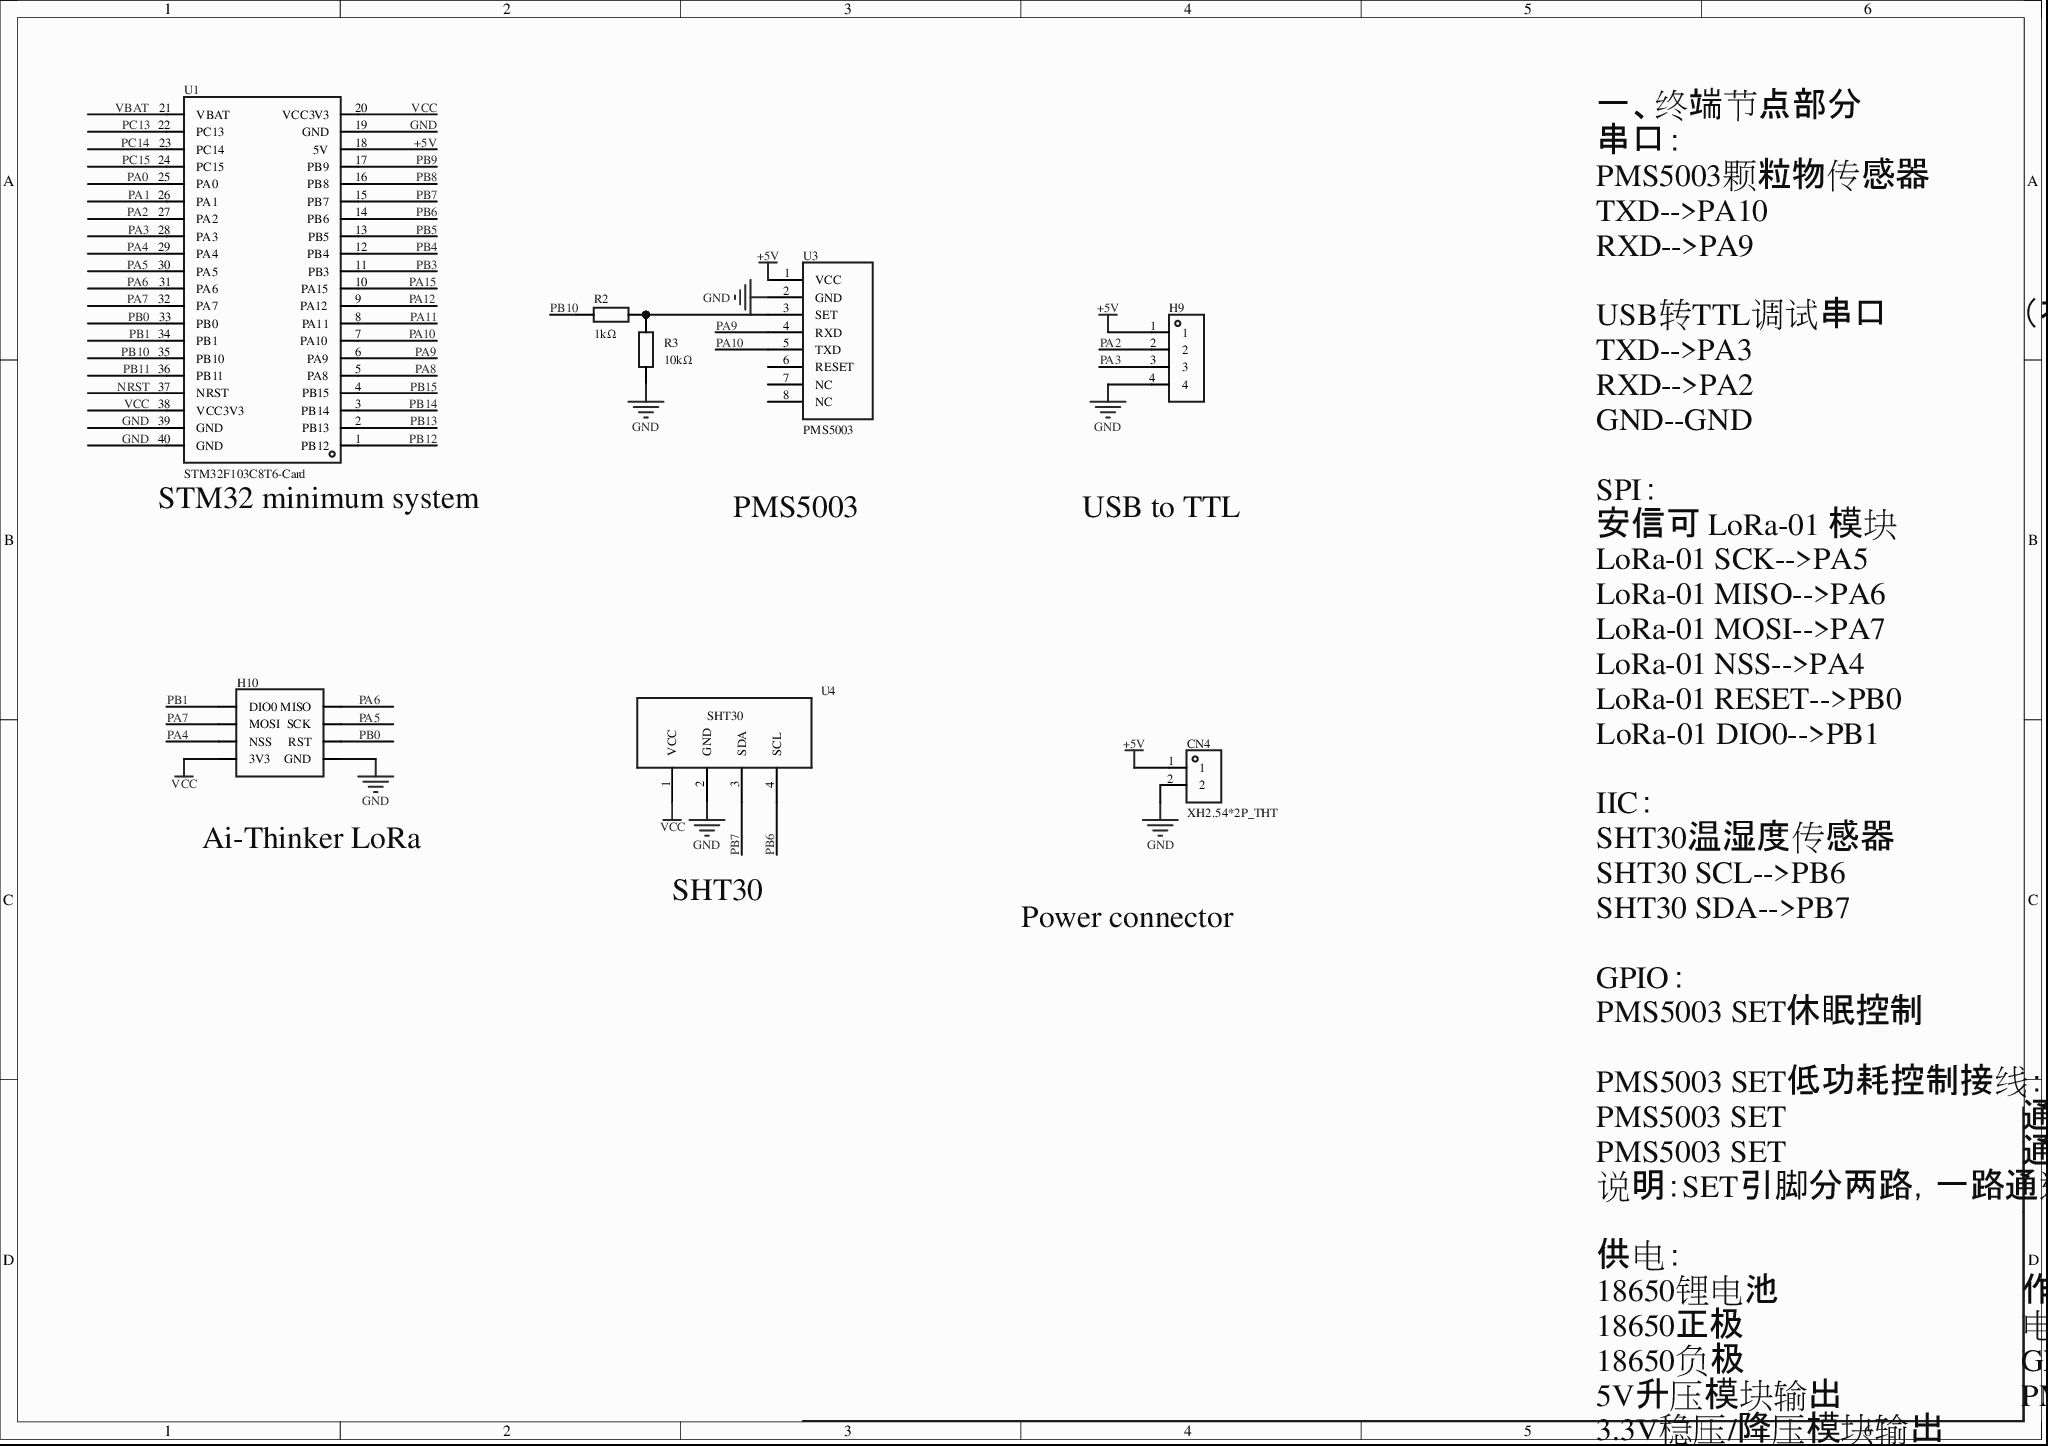
[diagram p0: MISC88998-3.schdoc]
# Altium project MISC88998-2.PrjPcb
1 sheet, 8 parts. Net scope: global (net labels, ports and power ports of the same name join across sheets).
Board file: MISC88998.pcbdoc

## Sheet MISC88998-3.schdoc
size 297 x 209 mm; Version: V1.0; @Project Name: MISC88998; @Page Count: 1; @Update Date: 2026-05-13; @Create Date: 2026-05-13; @Schematic Name: MISC88998; @Page No: 1; @Create Time: 23:22:16; @Update Time: 17:32:40; @Board Name: MISC88998

### Parts
CN4  XH2.54*2P_THT  [CONN-TH_2P-P2.50-XH2.54-2P]
H9  (no value)  [HDR-TH_4P-P2.54-V-M]
H10  (no value)  [HDR-TH_8P-P2.54-V-F-R2-C4-S2.54-1]
R2  1kΩ  [Res_1/8W]
R3  10kΩ  [Res_1/8W]
U1  STM32F103C8T6-Card  [CONN-TH_L53.3-W22.9_STM32F103C8T6-CARD]
U3  PMS5003  [1.25-LI-8P]
U4  (no value)  [SHT30模块]

### Nets
+5V: CN4.1 H9.1 U1.18(5V) U3.1(VCC)
GND: CN4.2 H9.4 H10.8(GND) R3.1 U1.19(GND) U1.39(GND) U1.40(GND) U3.2(GND) U4.2(GND)
VCC: H10.7(3V3) U1.20(VCC3V3) U1.38(VCC3V3) U4.1(VCC)
NRST: U1.37(NRST)
PA0: U1.25(PA0)
PA1: U1.26(PA1)
PA2: H9.2 U1.27(PA2)
PA3: H9.3 U1.28(PA3)
PA4: H10.5(NSS) U1.29(PA4)
PA5: H10.4(SCK) U1.30(PA5)
PA6: H10.2(MISO) U1.31(PA6)
PA7: H10.3(MOSI) U1.32(PA7)
PA8: U1.5(PA8)
PA9: U1.6(PA9) U3.4(RXD)
PA10: U1.7(PA10) U3.5(TXD)
PA11: U1.8(PA11)
PA12: U1.9(PA12)
PA15: U1.10(PA15)
PB0: H10.6(RST) U1.33(PB0)
PB1: H10.1(DIO0) U1.34(PB1)
PB3: U1.11(PB3)
PB4: U1.12(PB4)
PB5: U1.13(PB5)
PB6: U1.14(PB6) U4.4(SCL)
PB7: U1.15(PB7) U4.3(SDA)
PB8: U1.16(PB8)
PB9: U1.17(PB9)
PB10: R2.1 U1.35(PB10)
PB11: U1.36(PB11)
PB12: U1.1(PB12)
PB13: U1.2(PB13)
PB14: U1.3(PB14)
PB15: U1.4(PB15)
PC13: U1.22(PC13)
PC14: U1.23(PC14)
PC15: U1.24(PC15)
VBAT: U1.21(VBAT)
NetR2_2: R2.2 R3.2 U3.3(SET)

Not connected (* = marked no-connect by the designer): U3 6(RESET) 7(NC) 8(NC)

### Notes on the sheet
- 一、终端节点部分
  串口：
  PMS5003颗粒物传感器
  TXD-->PA10
  RXD-->PA9
  USB转TTL调试串口	（有单独模块不用画进PCB，给我留个接口即插即用）
  TXD-->PA3
  RXD-->PA2
  GND--GND
  SPI：
  安信可 LoRa-01 模块
  LoRa-01 SCK-->PA5
  LoRa-01 MISO-->PA6
  LoRa-01 MOSI-->PA7
  LoRa-01 NSS-->PA4
  LoRa-01 RESET-->PB0
  LoRa-01 DIO0-->PB1
  IIC：
  SHT30温湿度传感器
  SHT30 SCL-->PB6
  SHT30 SDA-->PB7
  GPIO：
  PMS5003 SET休眠控制		PB10
  PMS5003 SET低功耗控制接线：
  PMS5003 SET		通过1kΩ电阻接 STM32 PB10
  PMS5003 SET		通过10kΩ电阻接 GND
  说明：SET引脚分两路，一路通过1kΩ接PB10，另一路通过10kΩ接GND。PB10输出高电平时PMS5003工作，PB10输出低电平时PMS5003休眠；10kΩ下拉用于保证上电默认休眠。
  供电：
  18650锂电池		作为终端节点主电源
  18650正极		电源开关		系统电源输入
  18650负极		GND
  5V升压模块输出		PMS5003 VCC
  3.3V稳压/降压模块输出		STM32、SHT30、LoRa-01
  所有模块GND		公共GND
  说明：PMS5003由升压后的5V供电；STM32、SHT30和LoRa-01由稳定3.3V供电，LoRa-01不能接5V。
  电源滤波：
  LoRa-01 VCC 与 GND之间		并联10μF和0.1μF电容
  PMS5003 VCC 与 GND之间		并联100μF和0.1μF电容
  SWD下载接口：
  我的最小开发板上有，应该可以不用多做
- (near U1) STM32 minimum system
- PMS5003
- USB to TTL
- (near H10) Ai-Thinker LoRa
- SHT30
- Power connector

### Library data of the parts
CN4 = XH2.54*2P_直插: AddInBom: yes; ModelId: 325c595e30db4df8abe76612dd40b0fa0819f05c4eef4c71ace90d822a990e87; ModelTransform: 295.275,228.346,0,180,0,0,-0.002,-20.079,-137.795; Device: XH2.54*2P_THT; Symbol: XH2.54*2P_THT; FootprintName: CONN-TH_2P-P2.50-XH2.54-2P; LCSC Part Name: XH2.54*2P_直插; SupplierPart: C9900008615; ManufacturerPart: XH2.54*2P_直插; Supplier Footprint: XH2.54_2P; JLCPCB Part Class: Extended Part; Supplier: LCSC; ConvertToPcb: yes; ModelName: CONN-TH_2P-P2.50-XH2.54-2P
H9 = HDR-M_2.54_1x4P: Symbol: PZ254V-11-04P; ConvertToPcb: yes; ModelId: 112f4d05e8d64e99ab9a333894bea4f90819f05c4eef4c71ace90d822a990e87; ModelName: HDR-TH_4P-P2.54-M-LI-1X4P; ModelTransform: 399.999,104.7242,0,0,0,0,0,0,-118.11; Device: HDR-M_2.54_1x4P; AddInBom: yes; SupplierPart: C492403; Supplier Footprint: 插件; FootprintName: HDR-TH_4P-P2.54-V-M
H10 = HDR-F_2.54_2x4: Symbol: HDR-F-2.54_2x4; ConvertToPcb: yes; ModelId: 64729f32a5874cf59655d275a66f10500819f05c4eef4c71ace90d822a990e87; ModelName: HDR2.54-F-LI-2X4P; ModelTransform: 399.999,200,0,0,0,0,0,0,-118.11; Device: HDR-F_2.54_2x4; AddInBom: yes; SupplierPart: C92271; Supplier Footprint: 插件; FootprintName: HDR-TH_8P-P2.54-V-F-R2-C4-S2.54-1
R2 R3 = Res_AXIAL-1/8W: Symbol: Resistor; 3D Model: b2b5ae7ae4c642178fe0039925c86a3f0819f05c4eef4c71ace90d822a990e87; 3D Model Transform: 282.86,66.88,253.09,0,0,0,0,0,-191; ConvertToPcb: yes; ModelName: RES-TH_BD1.8-L3.2-P7.20-D0.4; Device: Res_AXIAL-1/8W; Supplier Footprint: 轴向引线; AddInBom: yes; FootprintName: Res_1/8W
  R2: Value: 1kΩ
  R3: Value: 10kΩ
U1 = STM32F103C8T6-Card: AddInBom: yes; Device: STM32F103C8T6-Card; Symbol: STM32F103C8T6-CARD; FootprintName: CONN-TH_L53.3-W22.9_STM32F103C8T6-CARD; LCSC Part Name: STM32F103C8T6-Card; SupplierPart: C9900077949; ManufacturerPart: STM32F103C8T6-Card; Supplier Footprint: 插件; Supplier: LCSC; ConvertToPcb: yes
U3 = PMS5003: ModelId: 8926deb8ee21459093e6f5db8bbe2de82760fa5781284a368d4cc4272a730d42; ModelTransform: 468.89,127.95,269.68,0,0,0,0,-18.900000000000002,-86.61; AddInBom: yes; Symbol: PMS5003; Device: PMS5003; FootprintName: 1.25-LI-8P; ModelName: 1.25-LI-8P; ConvertToPcb: yes
U4 = SHT30: AddInBom: yes; ModelId: edbf9416530e4d23b9398737350b1610fff7178baba14523b6c31c40b091539f; ModelName: SHT30 Dual Mounting Holes; ModelTransform: 472.4399880698992,721.65206,287.4009861719445,270,0,270,121.92913,122.12598,149.6063; Symbol: SHT30; Device: SHT30; ConvertToPcb: yes; FootprintName: SHT30 module